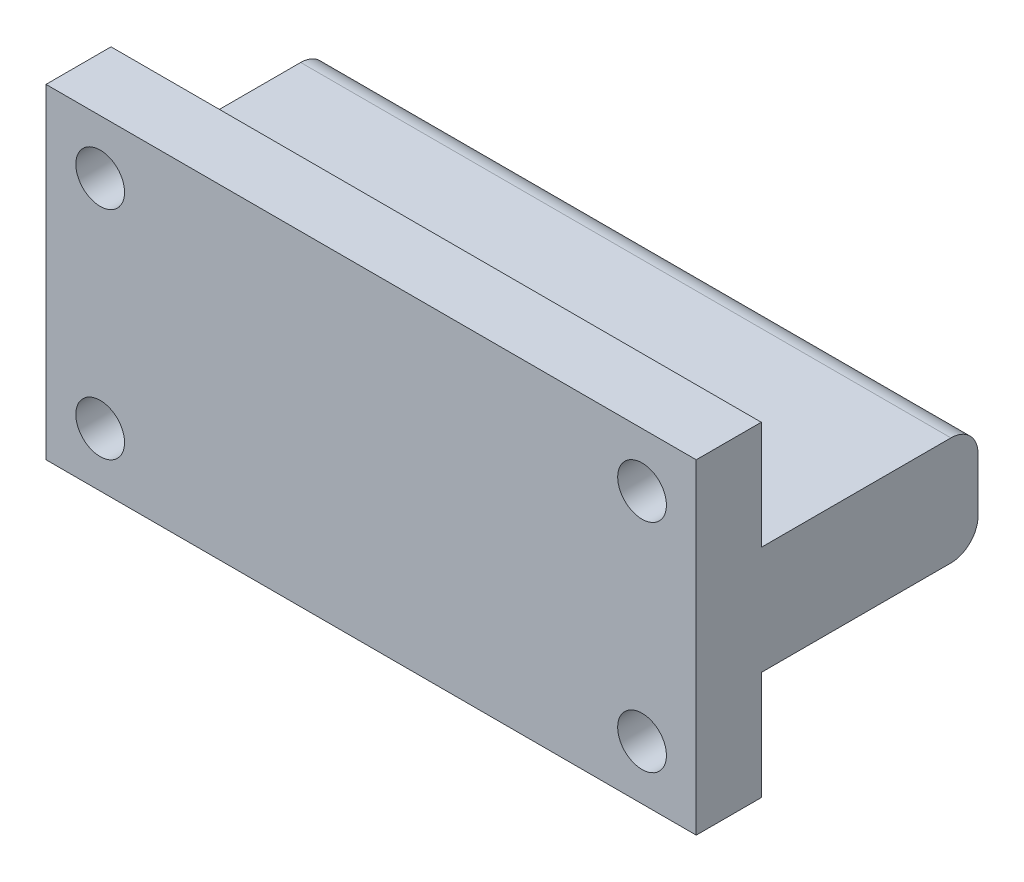
SolidWorks part; units mm, degrees
material "普通碳钢"
ref_plane "Front Plane" through (0, 0, 0) normal (0, 0, 1) x (1, 0, 0)
ref_plane "Top Plane" through (0, 0, 0) normal (0, 1, 0) x (1, 0, 0)
ref_plane "Right Plane" through (0, 0, 0) normal (1, 0, 0) x (0, 0, -1)
sketch "Sketch1" plane through (0, 0, 0) normal (0, 0, 1) x (1, 0, 0)
  line L1 (0, 0) -> (120, 0)
  line L2 (0, 0) -> (0, 60)
  line L3 (0, 60) -> (120, 60)
  line L4 (120, 0) -> (120, 60)
  dimension "D1" = 60
  dimension "D2" = 120
extrude "Boss-Extrude1" add sketch "Sketch1" along normal blind 12 contours L3 L4 L1 L2
hole_wizard "M6 Clearance Hole1" positions "Sketch4" profile "Sketch5" hole size "M6" standard "GB"
sketch "Sketch4" plane through (0, 0, 0) normal (0, 0, -1) x (-1, 0, 0)
  line L0 (-60, 60) -> (-60, 53.7197) construction
  line L1 (0, 60) -> (-120, 60) construction
  line L3 (-120, 30) -> (-122.9331, 30) construction
  line L4 (-120, 0) -> (-120, 60) construction
  point P0 (-110, 50)
  point P2 (-10, 50)
  point P4 (-10, 10)
  point P6 (-110, 10)
  dimension "D1" = 40
  dimension "D2" = 100
sketch "Sketch5" plane through (110, 50, 0) normal (1, 0, 0) x (0, 1, 0)
  line L0 (0, 0) -> (0, 35.4539)
  line L1 (0, 35.4539) -> (4.5, 32.75)
  line L2 (4.5, 32.75) -> (4.5, 0)
  line L5 (4.5, 0) -> (0, 0)
  line L10 (0, 35.4539) -> (-4.5, 32.75) construction
  line L11 (0, -6.35) -> (0, 107.95) construction
  dimension "孔直径" = 9
  dimension "孔深度" = 32.75
  dimension "导头角度" = 118
sketch "Sketch3" plane through (0, 0, 0) normal (0, 0, 1) x (1, 0, 0)
  line L0 (0, 30) -> (120, 30) construction
  line L1 (0, 0) -> (0, 60) construction
  line L2 (120, 0) -> (120, 60) construction
  line L4 (0, 40) -> (120, 40)
  line L5 (0, 40) -> (0, 20)
  line L6 (0, 20) -> (120, 20)
  line L7 (120, 40) -> (120, 20)
  line L8 (0, 40) -> (120, 20) construction
  line L9 (0, 20) -> (120, 40) construction
  point P6 (60, 30)
  dimension "D1" = 20
  dimension "D2" = 120
extrude "Boss-Extrude2" add sketch "Sketch3" against normal blind 40
fillet "Fillet1" radius 5 2 edges at (60, 40, -40) (60, 20, -40)
